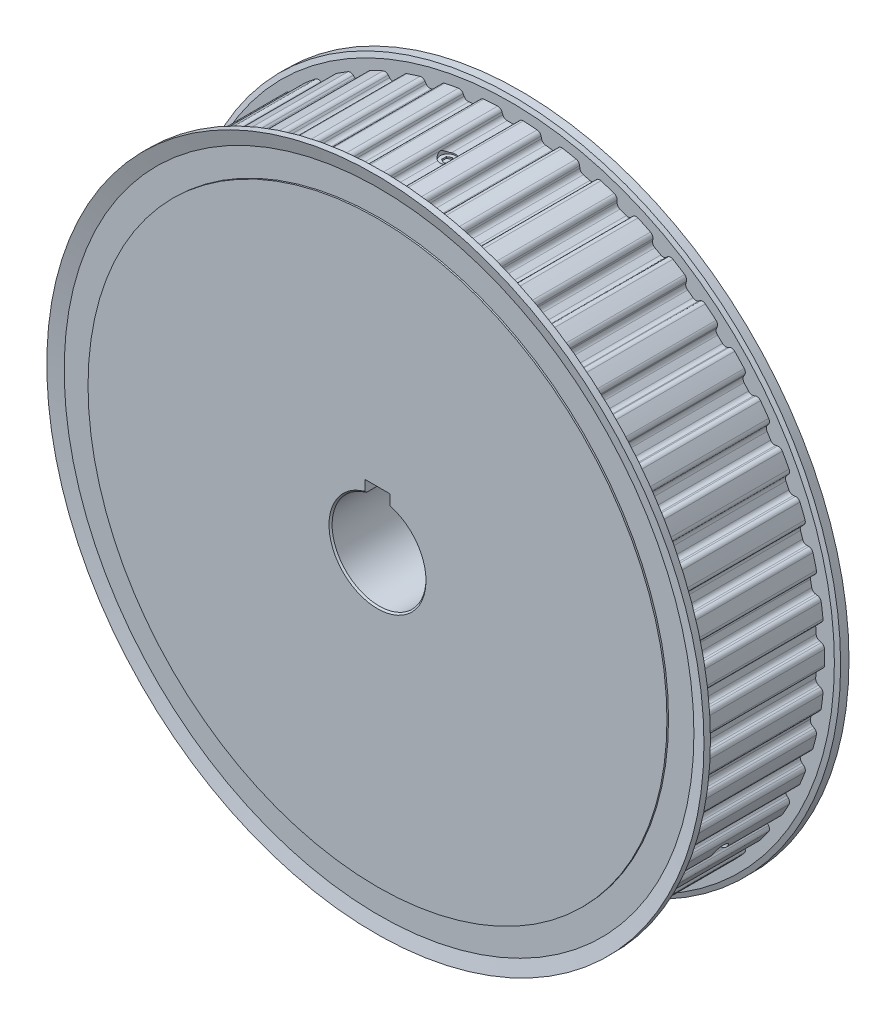
SolidWorks part; units mm, degrees
ref_plane "前视基准面" through (0, 0, 0) normal (0, 0, 1) x (1, 0, 0)
ref_plane "上视基准面" through (0, 0, 0) normal (0, 1, 0) x (1, 0, 0)
ref_plane "右视基准面" through (0, 0, 0) normal (1, 0, 0) x (0, 0, -1)
sketch "草图1" plane through (0, 0, 0) normal (1, 0, 0) x (0, 0, -1)
  line L0 (0, 0) -> (0, 92.5)
  line L1 (0, 92.5) -> (2.5, 92.5)
  line L2 (2.5, 92.5) -> (2.5, 102.38)
  line L3 (2.5, 102.38) -> (42.5, 102.38)
  line L4 (42.5, 102.38) -> (42.5, 92.5)
  line L5 (42.5, 92.5) -> (45, 92.5)
  line L6 (45, 92.5) -> (45, 0)
  line L7 (45, 0) -> (0, 0)
  line L8 (45, 0) -> (0, 0) construction
revolve "旋转1" add sketch "草图1" angle 360 about L8
sketch "草图2" plane through (0, 0, 0) normal (1, 0, 0) x (0, 0, -1)
  line L0 (0, 0) -> (0, 15.5)
  line L1 (0, 15.5) -> (0.5, 15)
  line L2 (0.5, 15) -> (44.5, 15)
  line L3 (44.5, 15) -> (45, 15.5)
  line L4 (45, 15.5) -> (45, 0)
  line L5 (45, 0) -> (0, 0)
  line L6 (45, 0) -> (0, 0) construction
revolve "切除-旋转1" cut sketch "草图2" angle 360 about L6
sketch "草图3" plane through (0, 0, 0) normal (1, 0, 0) x (0, 0, -1)
  line L0 (42.5, 103.5) -> (42.5, 92.5)
  line L1 (42.5, 92.5) -> (44.5, 92.5)
  line L2 (44.5, 92.5) -> (44.5, 105)
  line L3 (44.5, 105) -> (43, 105)
  line L4 (43, 105) -> (42.5, 103.5)
  line L5 (50, 0) -> (-50, 0) construction
revolve "旋转2" add sketch "草图3" angle 360 about L5
ref_plane "基准面1" through (0, 0, -22.5) normal (0, 0, 1) x (1, 0, 0)
sketch "草图4" plane through (0, 0, -22.5) normal (0, 0, 1) x (1, 0, 0)
  line L0 (-99.3369, -3.5434) -> (-98.7119, -3.7273)
  line L1 (-98.4007, -8.6739) -> (-98.9977, -8.9348)
  line L2 (-98.1095, -15.9657) -> (-97.4664, -16.0698)
  line L3 (-96.5376, -20.9384) -> (-97.0972, -21.272)
  line L4 (-95.3348, -28.1361) -> (-94.6838, -28.1589)
  line L5 (-93.1521, -32.8727) -> (-93.6655, -33.2738)
  line L6 (-91.0567, -39.8629) -> (-90.4079, -39.8039)
  line L7 (-88.2976, -44.2885) -> (-88.7566, -44.7508)
  line L8 (-85.3425, -50.961) -> (-84.7063, -50.8211)
  line L9 (-82.0505, -55.0059) -> (-82.448, -55.5221)
  line L10 (-78.2825, -61.2554) -> (-77.6687, -61.0369)
  line L11 (-74.5094, -64.8559) -> (-74.8391, -65.4178)
  line L12 (-69.9879, -70.5838) -> (-69.4064, -70.2901)
  line L13 (-65.7933, -73.683) -> (-66.0499, -74.2817)
  line L14 (-60.5895, -78.799) -> (-60.0494, -78.4347)
  line L15 (-56.0396, -81.348) -> (-56.2191, -81.9743)
  line L16 (-50.2356, -85.7715) -> (-49.7454, -85.3424)
  line L17 (-45.4021, -87.7302) -> (-45.5017, -88.374)
  line L18 (-39.0894, -91.3914) -> (-38.6569, -90.9042)
  line L19 (-34.0486, -92.7288) -> (-34.0667, -93.38)
  line L20 (-27.3268, -95.57) -> (-26.9588, -95.0324)
  line L21 (-22.1581, -96.265) -> (-22.0945, -96.9134)
  line L22 (-15.1333, -98.2413) -> (-14.8355, -97.6619)
  line L23 (-9.9181, -98.2831) -> (-9.7738, -98.9184)
  line L24 (-2.701, -99.3634) -> (-2.4782, -98.7512)
  line L25 (2.4782, -98.7512) -> (2.701, -99.3634)
  line L26 (9.7738, -98.9184) -> (9.9181, -98.2831)
  line L27 (14.8355, -97.6619) -> (15.1333, -98.2413)
  line L28 (22.0945, -96.9134) -> (22.1581, -96.265)
  line L29 (26.9588, -95.0324) -> (27.3268, -95.57)
  line L30 (34.0667, -93.38) -> (34.0486, -92.7288)
  line L31 (38.6569, -90.9042) -> (39.0894, -91.3914)
  line L32 (45.5017, -88.374) -> (45.4021, -87.7302)
  line L33 (49.7454, -85.3424) -> (50.2356, -85.7715)
  line L34 (56.2191, -81.9743) -> (56.0396, -81.348)
  line L35 (60.0494, -78.4347) -> (60.5895, -78.799)
  line L36 (66.0499, -74.2817) -> (65.7933, -73.683)
  line L37 (69.4064, -70.2901) -> (69.9879, -70.5838)
  line L38 (74.8391, -65.4178) -> (74.5094, -64.8559)
  line L39 (77.6687, -61.0369) -> (78.2825, -61.2554)
  line L40 (82.448, -55.5221) -> (82.0505, -55.0059)
  line L41 (84.7063, -50.8211) -> (85.3425, -50.961)
  line L42 (88.7566, -44.7508) -> (88.2976, -44.2885)
  line L43 (90.4079, -39.8039) -> (91.0567, -39.8629)
  line L44 (93.6655, -33.2738) -> (93.1521, -32.8727)
  line L45 (94.6838, -28.1589) -> (95.3348, -28.1361)
  line L46 (97.0972, -21.272) -> (96.5376, -20.9384)
  line L47 (97.4664, -16.0698) -> (98.1095, -15.9657)
  line L48 (98.9977, -8.9348) -> (98.4007, -8.6739)
  line L49 (98.7119, -3.7273) -> (99.3369, -3.5434)
  line L50 (99.3369, 3.5434) -> (98.7119, 3.7273)
  line L51 (98.4007, 8.6739) -> (98.9977, 8.9348)
  line L52 (98.1095, 15.9657) -> (97.4664, 16.0698)
  line L53 (96.5376, 20.9384) -> (97.0972, 21.272)
  line L54 (95.3348, 28.1361) -> (94.6838, 28.1589)
  line L55 (93.1521, 32.8727) -> (93.6655, 33.2738)
  line L56 (91.0567, 39.8629) -> (90.4079, 39.8039)
  line L57 (88.2976, 44.2885) -> (88.7566, 44.7508)
  line L58 (85.3425, 50.961) -> (84.7063, 50.8211)
  line L59 (82.0505, 55.0059) -> (82.448, 55.5221)
  line L60 (78.2825, 61.2554) -> (77.6687, 61.0369)
  line L61 (74.5094, 64.8559) -> (74.8391, 65.4178)
  line L62 (69.9879, 70.5838) -> (69.4064, 70.2901)
  line L63 (65.7933, 73.683) -> (66.0499, 74.2817)
  line L64 (60.5895, 78.799) -> (60.0494, 78.4347)
  line L65 (56.0396, 81.348) -> (56.2191, 81.9743)
  line L66 (50.2356, 85.7715) -> (49.7454, 85.3424)
  line L67 (45.4021, 87.7302) -> (45.5017, 88.374)
  line L68 (39.0894, 91.3914) -> (38.6569, 90.9042)
  line L69 (34.0486, 92.7288) -> (34.0667, 93.38)
  line L70 (27.3268, 95.57) -> (26.9588, 95.0324)
  line L71 (22.1581, 96.265) -> (22.0945, 96.9134)
  line L72 (15.1333, 98.2413) -> (14.8355, 97.6619)
  line L73 (9.9181, 98.2831) -> (9.7738, 98.9184)
  line L74 (2.701, 99.3634) -> (2.4782, 98.7512)
  line L75 (-2.4782, 98.7512) -> (-2.701, 99.3634)
  line L76 (-9.7738, 98.9184) -> (-9.9181, 98.2831)
  line L77 (-14.8355, 97.6619) -> (-15.1333, 98.2413)
  line L78 (-22.0945, 96.9134) -> (-22.1581, 96.265)
  line L79 (-26.9588, 95.0324) -> (-27.3268, 95.57)
  line L80 (-34.0667, 93.38) -> (-34.0486, 92.7288)
  line L81 (-38.6569, 90.9042) -> (-39.0894, 91.3914)
  line L82 (-45.5017, 88.374) -> (-45.4021, 87.7302)
  line L83 (-49.7454, 85.3424) -> (-50.2356, 85.7715)
  line L84 (-56.2191, 81.9743) -> (-56.0396, 81.348)
  line L85 (-60.0494, 78.4347) -> (-60.5895, 78.799)
  line L86 (-66.0499, 74.2817) -> (-65.7933, 73.683)
  line L87 (-69.4064, 70.2901) -> (-69.9879, 70.5838)
  line L88 (-74.8391, 65.4178) -> (-74.5094, 64.8559)
  line L89 (-77.6687, 61.0369) -> (-78.2825, 61.2554)
  line L90 (-82.448, 55.5221) -> (-82.0505, 55.0059)
  line L91 (-84.7063, 50.8211) -> (-85.3425, 50.961)
  line L92 (-88.7566, 44.7508) -> (-88.2976, 44.2885)
  line L93 (-90.4079, 39.8039) -> (-91.0567, 39.8629)
  line L94 (-93.6655, 33.2738) -> (-93.1521, 32.8727)
  line L95 (-94.6838, 28.1589) -> (-95.3348, 28.1361)
  line L96 (-97.0972, 21.272) -> (-96.5376, 20.9384)
  line L97 (-97.4664, 16.0698) -> (-98.1095, 15.9657)
  line L98 (-98.9977, 8.9348) -> (-98.4007, 8.6739)
  line L99 (-98.7119, 3.7273) -> (-99.3369, 3.5434)
  circle A0 centre (0, 0) radius 200.76
  arc A1 (-100.3556, 2.2125) -> (-100.3556, -2.2125) centre (0, 0) ccw
  arc A2 (-100.3556, -2.2125) -> (-99.3369, -3.5434) centre (-98.936, -2.1812) ccw
  arc A3 (-98.7119, -3.7273) -> (-97.6589, -5.0614) centre (-99.127, -5.1375) cw
  arc A4 (-97.6589, -5.0614) -> (-97.5232, -7.2184) centre (0, 0) ccw
  arc A5 (-97.5232, -7.2184) -> (-98.4007, -8.6739) centre (-98.9892, -7.3269) cw
  arc A6 (-98.9977, -8.9348) -> (-99.8416, -10.3829) centre (-98.4292, -10.236) ccw
  arc A7 (-99.8416, -10.3829) -> (-99.287, -14.7729) centre (0, 0) ccw
  arc A8 (-99.287, -14.7729) -> (-98.1095, -15.9657) centre (-97.8824, -14.5639) ccw
  arc A9 (-97.4664, -16.0698) -> (-96.2545, -17.2614) centre (-97.7014, -17.5209) cw
  arc A10 (-96.2545, -17.2614) -> (-95.8495, -19.3844) centre (0, 0) ccw
  arc A11 (-95.8495, -19.3844) -> (-96.5376, -20.9384) centre (-97.2903, -19.6758) cw
  arc A12 (-97.0972, -21.272) -> (-97.753, -22.8145) centre (-96.3701, -22.4917) ccw
  arc A13 (-97.753, -22.8145) -> (-96.6525, -27.1004) centre (0, 0) ccw
  arc A14 (-96.6525, -27.1004) -> (-95.3348, -28.1361) centre (-95.2853, -26.717) ccw
  arc A15 (-94.6838, -28.1589) -> (-93.3321, -29.1892) centre (-94.7351, -29.628) cw
  arc A16 (-93.3321, -29.1892) -> (-92.6642, -31.2446) centre (0, 0) ccw
  arc A17 (-92.6642, -31.2446) -> (-93.1521, -32.8727) centre (-94.0572, -31.7143) cw
  arc A18 (-93.6655, -33.2738) -> (-94.1228, -34.8863) centre (-92.7913, -34.3928) ccw
  arc A19 (-94.1228, -34.8863) -> (-92.4938, -39.0005) centre (0, 0) ccw
  arc A20 (-92.4938, -39.0005) -> (-91.0567, -39.8629) centre (-91.1854, -38.4487) ccw
  arc A21 (-90.4079, -39.8039) -> (-88.9377, -40.6566) centre (-90.2747, -41.2678) cw
  arc A22 (-88.9377, -40.6566) -> (-88.0175, -42.6122) centre (0, 0) ccw
  arc A23 (-88.0175, -42.6122) -> (-88.2976, -44.2885) centre (-89.3406, -43.2527) cw
  arc A24 (-88.7566, -44.7508) -> (-89.0082, -46.4079) centre (-87.749, -45.7514) ccw
  arc A25 (-89.0082, -46.4079) -> (-86.8764, -50.2855) centre (0, 0) ccw
  arc A26 (-86.8764, -50.2855) -> (-85.3425, -50.961) centre (-85.6475, -49.5741) ccw
  arc A27 (-84.7063, -50.8211) -> (-83.1408, -51.4829) centre (-84.3906, -52.2568) cw
  arc A28 (-83.1408, -51.4829) -> (-81.9828, -53.3077) centre (0, 0) ccw
  arc A29 (-81.9828, -53.3077) -> (-82.0505, -55.0059) centre (-83.2151, -54.109) cw
  arc A30 (-82.448, -55.5221) -> (-82.4898, -57.1976) centre (-81.3229, -56.3885) ccw
  arc A31 (-82.4898, -57.1976) -> (-79.8889, -60.7775) centre (0, 0) ccw
  arc A32 (-79.8889, -60.7775) -> (-78.2825, -61.2554) centre (-78.7588, -59.9177) ccw
  arc A33 (-77.6687, -61.0369) -> (-76.0327, -61.4973) centre (-77.1756, -62.4217) cw
  arc A34 (-76.0327, -61.4973) -> (-74.6551, -63.1625) centre (0, 0) ccw
  arc A35 (-74.6551, -63.1625) -> (-74.5094, -64.8559) centre (-75.7773, -64.112) cw
  arc A36 (-74.8391, -65.4178) -> (-74.6706, -67.0853) centre (-73.6143, -66.1363) ccw
  arc A37 (-74.6706, -67.0853) -> (-71.6416, -70.311) centre (0, 0) ccw
  arc A38 (-71.6416, -70.311) -> (-69.9879, -70.5838) centre (-70.6281, -69.3163) ccw
  arc A39 (-69.4064, -70.2901) -> (-67.7255, -70.5418) centre (-68.7436, -71.6022) cw
  arc A40 (-67.7255, -70.5418) -> (-66.15, -72.0212) centre (0, 0) ccw
  arc A41 (-66.15, -72.0212) -> (-65.7933, -73.683) centre (-67.1444, -73.1039) cw
  arc A42 (-66.0499, -74.2817) -> (-65.6738, -75.9151) centre (-64.7448, -74.8411) ccw
  arc A43 (-65.6738, -75.9151) -> (-62.2643, -78.7356) centre (0, 0) ccw
  arc A44 (-62.2643, -78.7356) -> (-60.5895, -78.799) centre (-61.3835, -77.6218) ccw
  arc A45 (-60.0494, -78.4347) -> (-58.3502, -78.4738) centre (-59.2274, -79.6534) cw
  arc A46 (-58.3502, -78.4738) -> (-56.6018, -79.7441) centre (0, 0) ccw
  arc A47 (-56.6018, -79.7441) -> (-56.0396, -81.348) centre (-57.4526, -80.9428) cw
  arc A48 (-56.2191, -81.9743) -> (-55.6413, -83.5476) centre (-54.8542, -82.3657) ccw
  arc A49 (-55.6413, -83.5476) -> (-51.9052, -85.9185) centre (0, 0) ccw
  arc A50 (-51.9052, -85.9185) -> (-50.2356, -85.7715) centre (-51.1709, -84.7031) ccw
  arc A51 (-49.7454, -85.3424) -> (-48.0548, -85.1682) centre (-48.7771, -86.4485) cw
  arc A52 (-48.0548, -85.1682) -> (-46.1609, -86.2094) centre (0, 0) ccw
  arc A53 (-46.1609, -86.2094) -> (-45.4021, -87.7302) centre (-46.8548, -87.5053) cw
  arc A54 (-45.5017, -88.374) -> (-44.7312, -89.8625) centre (-44.0985, -88.5912) ccw
  arc A55 (-44.7312, -89.8625) -> (-40.7275, -91.7465) centre (0, 0) ccw
  arc A56 (-40.7275, -91.7465) -> (-39.0894, -91.3914) centre (-40.1513, -90.4486) ccw
  arc A57 (-38.6569, -90.9042) -> (-37.0014, -90.5195) centre (-37.5576, -91.8802) cw
  arc A58 (-37.0014, -90.5195) -> (-34.992, -91.3151) centre (0, 0) ccw
  arc A59 (-34.992, -91.3151) -> (-34.0486, -92.7288) centre (-35.518, -92.6878) cw
  arc A60 (-34.0667, -93.38) -> (-33.1158, -94.7602) centre (-32.6473, -93.4197) ccw
  arc A61 (-33.1158, -94.7602) -> (-28.9074, -96.1275) centre (0, 0) ccw
  arc A62 (-28.9074, -96.1275) -> (-27.3268, -95.57) centre (-28.4985, -94.7677) ccw
  arc A63 (-26.9588, -95.0324) -> (-25.3646, -94.4432) centre (-25.7458, -95.8629) cw
  arc A64 (-25.3646, -94.4432) -> (-23.2712, -94.9807) centre (0, 0) ccw
  arc A65 (-23.2712, -94.9807) -> (-22.1581, -96.265) centre (-23.6211, -96.4085) cw
  arc A66 (-22.0945, -96.9134) -> (-20.978, -98.1635) centre (-20.6813, -96.7748) ccw
  arc A67 (-20.978, -98.1635) -> (-16.6315, -98.9926) centre (0, 0) ccw
  arc A68 (-16.6315, -98.9926) -> (-15.1333, -98.2413) centre (-16.3962, -97.5922) ccw
  arc A69 (-14.8355, -97.6619) -> (-13.3277, -96.8775) centre (-13.528, -98.3338) cw
  arc A70 (-13.3277, -96.8775) -> (-11.1835, -97.1484) centre (0, 0) ccw
  arc A71 (-11.1835, -97.1484) -> (-9.9181, -98.2831) centre (-11.3516, -98.6088) cw
  arc A72 (-9.7738, -98.9184) -> (-8.5095, -100.0187) centre (-8.3891, -98.6038) ccw
  arc A73 (-8.5095, -100.0187) -> (-4.0933, -100.2965) centre (0, 0) ccw
  arc A74 (-4.0933, -100.2965) -> (-2.701, -99.3634) centre (-4.0354, -98.8777) ccw
  arc A75 (-2.4782, -98.7512) -> (-1.0806, -97.784) centre (-1.0969, -99.2539) cw
  arc A76 (-1.0806, -97.784) -> (1.0806, -97.784) centre (0, 0) ccw
  arc A77 (1.0806, -97.784) -> (2.4782, -98.7512) centre (1.0969, -99.2539) cw
  arc A78 (2.701, -99.3634) -> (4.0933, -100.2965) centre (4.0354, -98.8777) ccw
  arc A79 (4.0933, -100.2965) -> (8.5095, -100.0187) centre (0, 0) ccw
  arc A80 (8.5095, -100.0187) -> (9.7738, -98.9184) centre (8.3891, -98.6038) ccw
  arc A81 (9.9181, -98.2831) -> (11.1835, -97.1484) centre (11.3516, -98.6088) cw
  arc A82 (11.1835, -97.1484) -> (13.3277, -96.8775) centre (0, 0) ccw
  arc A83 (13.3277, -96.8775) -> (14.8355, -97.6619) centre (13.528, -98.3338) cw
  arc A84 (15.1333, -98.2413) -> (16.6315, -98.9926) centre (16.3962, -97.5922) ccw
  arc A85 (16.6315, -98.9926) -> (20.978, -98.1635) centre (0, 0) ccw
  arc A86 (20.978, -98.1635) -> (22.0945, -96.9134) centre (20.6813, -96.7748) ccw
  arc A87 (22.1581, -96.265) -> (23.2712, -94.9807) centre (23.6211, -96.4085) cw
  arc A88 (23.2712, -94.9807) -> (25.3646, -94.4432) centre (0, 0) ccw
  arc A89 (25.3646, -94.4432) -> (26.9588, -95.0324) centre (25.7458, -95.8629) cw
  arc A90 (27.3268, -95.57) -> (28.9074, -96.1275) centre (28.4985, -94.7677) ccw
  arc A91 (28.9074, -96.1275) -> (33.1158, -94.7602) centre (0, 0) ccw
  arc A92 (33.1158, -94.7602) -> (34.0667, -93.38) centre (32.6473, -93.4197) ccw
  arc A93 (34.0486, -92.7288) -> (34.992, -91.3151) centre (35.518, -92.6878) cw
  arc A94 (34.992, -91.3151) -> (37.0014, -90.5195) centre (0, 0) ccw
  arc A95 (37.0014, -90.5195) -> (38.6569, -90.9042) centre (37.5576, -91.8802) cw
  arc A96 (39.0894, -91.3914) -> (40.7275, -91.7465) centre (40.1513, -90.4486) ccw
  arc A97 (40.7275, -91.7465) -> (44.7312, -89.8625) centre (0, 0) ccw
  arc A98 (44.7312, -89.8625) -> (45.5017, -88.374) centre (44.0985, -88.5912) ccw
  arc A99 (45.4021, -87.7302) -> (46.1609, -86.2094) centre (46.8548, -87.5053) cw
  arc A100 (46.1609, -86.2094) -> (48.0548, -85.1682) centre (0, 0) ccw
  arc A101 (48.0548, -85.1682) -> (49.7454, -85.3424) centre (48.7771, -86.4485) cw
  arc A102 (50.2356, -85.7715) -> (51.9052, -85.9185) centre (51.1709, -84.7031) ccw
  arc A103 (51.9052, -85.9185) -> (55.6413, -83.5476) centre (0, 0) ccw
  arc A104 (55.6413, -83.5476) -> (56.2191, -81.9743) centre (54.8542, -82.3657) ccw
  arc A105 (56.0396, -81.348) -> (56.6018, -79.7441) centre (57.4526, -80.9428) cw
  arc A106 (56.6018, -79.7441) -> (58.3502, -78.4738) centre (0, 0) ccw
  arc A107 (58.3502, -78.4738) -> (60.0494, -78.4347) centre (59.2274, -79.6534) cw
  arc A108 (60.5895, -78.799) -> (62.2643, -78.7356) centre (61.3835, -77.6218) ccw
  arc A109 (62.2643, -78.7356) -> (65.6738, -75.9151) centre (0, 0) ccw
  arc A110 (65.6738, -75.9151) -> (66.0499, -74.2817) centre (64.7448, -74.8411) ccw
  arc A111 (65.7933, -73.683) -> (66.15, -72.0212) centre (67.1444, -73.1039) cw
  arc A112 (66.15, -72.0212) -> (67.7255, -70.5418) centre (0, 0) ccw
  arc A113 (67.7255, -70.5418) -> (69.4064, -70.2901) centre (68.7436, -71.6022) cw
  arc A114 (69.9879, -70.5838) -> (71.6416, -70.311) centre (70.6281, -69.3163) ccw
  arc A115 (71.6416, -70.311) -> (74.6706, -67.0853) centre (0, 0) ccw
  arc A116 (74.6706, -67.0853) -> (74.8391, -65.4178) centre (73.6143, -66.1363) ccw
  arc A117 (74.5094, -64.8559) -> (74.6551, -63.1625) centre (75.7773, -64.112) cw
  arc A118 (74.6551, -63.1625) -> (76.0327, -61.4973) centre (0, 0) ccw
  arc A119 (76.0327, -61.4973) -> (77.6687, -61.0369) centre (77.1756, -62.4217) cw
  arc A120 (78.2825, -61.2554) -> (79.8889, -60.7775) centre (78.7588, -59.9177) ccw
  arc A121 (79.8889, -60.7775) -> (82.4898, -57.1976) centre (0, 0) ccw
  arc A122 (82.4898, -57.1976) -> (82.448, -55.5221) centre (81.3229, -56.3885) ccw
  arc A123 (82.0505, -55.0059) -> (81.9828, -53.3077) centre (83.2151, -54.109) cw
  arc A124 (81.9828, -53.3077) -> (83.1408, -51.4829) centre (0, 0) ccw
  arc A125 (83.1408, -51.4829) -> (84.7063, -50.8211) centre (84.3906, -52.2568) cw
  arc A126 (85.3425, -50.961) -> (86.8764, -50.2855) centre (85.6475, -49.5741) ccw
  arc A127 (86.8764, -50.2855) -> (89.0082, -46.4079) centre (0, 0) ccw
  arc A128 (89.0082, -46.4079) -> (88.7566, -44.7508) centre (87.749, -45.7514) ccw
  arc A129 (88.2976, -44.2885) -> (88.0175, -42.6122) centre (89.3406, -43.2527) cw
  arc A130 (88.0175, -42.6122) -> (88.9377, -40.6566) centre (0, 0) ccw
  arc A131 (88.9377, -40.6566) -> (90.4079, -39.8039) centre (90.2747, -41.2678) cw
  arc A132 (91.0567, -39.8629) -> (92.4938, -39.0005) centre (91.1854, -38.4487) ccw
  arc A133 (92.4938, -39.0005) -> (94.1228, -34.8863) centre (0, 0) ccw
  arc A134 (94.1228, -34.8863) -> (93.6655, -33.2738) centre (92.7913, -34.3928) ccw
  arc A135 (93.1521, -32.8727) -> (92.6642, -31.2446) centre (94.0572, -31.7143) cw
  arc A136 (92.6642, -31.2446) -> (93.3321, -29.1892) centre (0, 0) ccw
  arc A137 (93.3321, -29.1892) -> (94.6838, -28.1589) centre (94.7351, -29.628) cw
  arc A138 (95.3348, -28.1361) -> (96.6525, -27.1004) centre (95.2853, -26.717) ccw
  arc A139 (96.6525, -27.1004) -> (97.753, -22.8145) centre (0, 0) ccw
  arc A140 (97.753, -22.8145) -> (97.0972, -21.272) centre (96.3701, -22.4917) ccw
  arc A141 (96.5376, -20.9384) -> (95.8495, -19.3844) centre (97.2903, -19.6758) cw
  arc A142 (95.8495, -19.3844) -> (96.2545, -17.2614) centre (0, 0) ccw
  arc A143 (96.2545, -17.2614) -> (97.4664, -16.0698) centre (97.7014, -17.5209) cw
  arc A144 (98.1095, -15.9657) -> (99.287, -14.7729) centre (97.8824, -14.5639) ccw
  arc A145 (99.287, -14.7729) -> (99.8416, -10.3829) centre (0, 0) ccw
  arc A146 (99.8416, -10.3829) -> (98.9977, -8.9348) centre (98.4292, -10.236) ccw
  arc A147 (98.4007, -8.6739) -> (97.5232, -7.2184) centre (98.9892, -7.3269) cw
  arc A148 (97.5232, -7.2184) -> (97.6589, -5.0614) centre (0, 0) ccw
  arc A149 (97.6589, -5.0614) -> (98.7119, -3.7273) centre (99.127, -5.1375) cw
  arc A150 (99.3369, -3.5434) -> (100.3556, -2.2125) centre (98.936, -2.1812) ccw
  arc A151 (100.3556, -2.2125) -> (100.3556, 2.2125) centre (0, 0) ccw
  arc A152 (100.3556, 2.2125) -> (99.3369, 3.5434) centre (98.936, 2.1812) ccw
  arc A153 (98.7119, 3.7273) -> (97.6589, 5.0614) centre (99.127, 5.1375) cw
  arc A154 (97.6589, 5.0614) -> (97.5232, 7.2184) centre (0, 0) ccw
  arc A155 (97.5232, 7.2184) -> (98.4007, 8.6739) centre (98.9892, 7.3269) cw
  arc A156 (98.9977, 8.9348) -> (99.8416, 10.3829) centre (98.4292, 10.236) ccw
  arc A157 (99.8416, 10.3829) -> (99.287, 14.7729) centre (0, 0) ccw
  arc A158 (99.287, 14.7729) -> (98.1095, 15.9657) centre (97.8824, 14.5639) ccw
  arc A159 (97.4664, 16.0698) -> (96.2545, 17.2614) centre (97.7014, 17.5209) cw
  arc A160 (96.2545, 17.2614) -> (95.8495, 19.3844) centre (0, 0) ccw
  arc A161 (95.8495, 19.3844) -> (96.5376, 20.9384) centre (97.2903, 19.6758) cw
  arc A162 (97.0972, 21.272) -> (97.753, 22.8145) centre (96.3701, 22.4917) ccw
  arc A163 (97.753, 22.8145) -> (96.6525, 27.1004) centre (0, 0) ccw
  arc A164 (96.6525, 27.1004) -> (95.3348, 28.1361) centre (95.2853, 26.717) ccw
  arc A165 (94.6838, 28.1589) -> (93.3321, 29.1892) centre (94.7351, 29.628) cw
  arc A166 (93.3321, 29.1892) -> (92.6642, 31.2446) centre (0, 0) ccw
  arc A167 (92.6642, 31.2446) -> (93.1521, 32.8727) centre (94.0572, 31.7143) cw
  arc A168 (93.6655, 33.2738) -> (94.1228, 34.8863) centre (92.7913, 34.3928) ccw
  arc A169 (94.1228, 34.8863) -> (92.4938, 39.0005) centre (0, 0) ccw
  arc A170 (92.4938, 39.0005) -> (91.0567, 39.8629) centre (91.1854, 38.4487) ccw
  arc A171 (90.4079, 39.8039) -> (88.9377, 40.6566) centre (90.2747, 41.2678) cw
  arc A172 (88.9377, 40.6566) -> (88.0175, 42.6122) centre (0, 0) ccw
  arc A173 (88.0175, 42.6122) -> (88.2976, 44.2885) centre (89.3406, 43.2527) cw
  arc A174 (88.7566, 44.7508) -> (89.0082, 46.4079) centre (87.749, 45.7514) ccw
  arc A175 (89.0082, 46.4079) -> (86.8764, 50.2855) centre (0, 0) ccw
  arc A176 (86.8764, 50.2855) -> (85.3425, 50.961) centre (85.6475, 49.5741) ccw
  arc A177 (84.7063, 50.8211) -> (83.1408, 51.4829) centre (84.3906, 52.2568) cw
  arc A178 (83.1408, 51.4829) -> (81.9828, 53.3077) centre (0, 0) ccw
  arc A179 (81.9828, 53.3077) -> (82.0505, 55.0059) centre (83.2151, 54.109) cw
  arc A180 (82.448, 55.5221) -> (82.4898, 57.1976) centre (81.3229, 56.3885) ccw
  arc A181 (82.4898, 57.1976) -> (79.8889, 60.7775) centre (0, 0) ccw
  arc A182 (79.8889, 60.7775) -> (78.2825, 61.2554) centre (78.7588, 59.9177) ccw
  arc A183 (77.6687, 61.0369) -> (76.0327, 61.4973) centre (77.1756, 62.4217) cw
  arc A184 (76.0327, 61.4973) -> (74.6551, 63.1625) centre (0, 0) ccw
  arc A185 (74.6551, 63.1625) -> (74.5094, 64.8559) centre (75.7773, 64.112) cw
  arc A186 (74.8391, 65.4178) -> (74.6706, 67.0853) centre (73.6143, 66.1363) ccw
  arc A187 (74.6706, 67.0853) -> (71.6416, 70.311) centre (0, 0) ccw
  arc A188 (71.6416, 70.311) -> (69.9879, 70.5838) centre (70.6281, 69.3163) ccw
  arc A189 (69.4064, 70.2901) -> (67.7255, 70.5418) centre (68.7436, 71.6022) cw
  arc A190 (67.7255, 70.5418) -> (66.15, 72.0212) centre (0, 0) ccw
  arc A191 (66.15, 72.0212) -> (65.7933, 73.683) centre (67.1444, 73.1039) cw
  arc A192 (66.0499, 74.2817) -> (65.6738, 75.9151) centre (64.7448, 74.8411) ccw
  arc A193 (65.6738, 75.9151) -> (62.2643, 78.7356) centre (0, 0) ccw
  arc A194 (62.2643, 78.7356) -> (60.5895, 78.799) centre (61.3835, 77.6218) ccw
  arc A195 (60.0494, 78.4347) -> (58.3502, 78.4738) centre (59.2274, 79.6534) cw
  arc A196 (58.3502, 78.4738) -> (56.6018, 79.7441) centre (0, 0) ccw
  arc A197 (56.6018, 79.7441) -> (56.0396, 81.348) centre (57.4526, 80.9428) cw
  arc A198 (56.2191, 81.9743) -> (55.6413, 83.5476) centre (54.8542, 82.3657) ccw
  arc A199 (55.6413, 83.5476) -> (51.9052, 85.9185) centre (0, 0) ccw
  arc A200 (51.9052, 85.9185) -> (50.2356, 85.7715) centre (51.1709, 84.7031) ccw
  arc A201 (49.7454, 85.3424) -> (48.0548, 85.1682) centre (48.7771, 86.4485) cw
  arc A202 (48.0548, 85.1682) -> (46.1609, 86.2094) centre (0, 0) ccw
  arc A203 (46.1609, 86.2094) -> (45.4021, 87.7302) centre (46.8548, 87.5053) cw
  arc A204 (45.5017, 88.374) -> (44.7312, 89.8625) centre (44.0985, 88.5912) ccw
  arc A205 (44.7312, 89.8625) -> (40.7275, 91.7465) centre (0, 0) ccw
  arc A206 (40.7275, 91.7465) -> (39.0894, 91.3914) centre (40.1513, 90.4486) ccw
  arc A207 (38.6569, 90.9042) -> (37.0014, 90.5195) centre (37.5576, 91.8802) cw
  arc A208 (37.0014, 90.5195) -> (34.992, 91.3151) centre (0, 0) ccw
  arc A209 (34.992, 91.3151) -> (34.0486, 92.7288) centre (35.518, 92.6878) cw
  arc A210 (34.0667, 93.38) -> (33.1158, 94.7602) centre (32.6473, 93.4197) ccw
  arc A211 (33.1158, 94.7602) -> (28.9074, 96.1275) centre (0, 0) ccw
  arc A212 (28.9074, 96.1275) -> (27.3268, 95.57) centre (28.4985, 94.7677) ccw
  arc A213 (26.9588, 95.0324) -> (25.3646, 94.4432) centre (25.7458, 95.8629) cw
  arc A214 (25.3646, 94.4432) -> (23.2712, 94.9807) centre (0, 0) ccw
  arc A215 (23.2712, 94.9807) -> (22.1581, 96.265) centre (23.6211, 96.4085) cw
  arc A216 (22.0945, 96.9134) -> (20.978, 98.1635) centre (20.6813, 96.7748) ccw
  arc A217 (20.978, 98.1635) -> (16.6315, 98.9926) centre (0, 0) ccw
  arc A218 (16.6315, 98.9926) -> (15.1333, 98.2413) centre (16.3962, 97.5922) ccw
  arc A219 (14.8355, 97.6619) -> (13.3277, 96.8775) centre (13.528, 98.3338) cw
  arc A220 (13.3277, 96.8775) -> (11.1835, 97.1484) centre (0, 0) ccw
  arc A221 (11.1835, 97.1484) -> (9.9181, 98.2831) centre (11.3516, 98.6088) cw
  arc A222 (9.7738, 98.9184) -> (8.5095, 100.0187) centre (8.3891, 98.6038) ccw
  arc A223 (8.5095, 100.0187) -> (4.0933, 100.2965) centre (0, 0) ccw
  arc A224 (4.0933, 100.2965) -> (2.701, 99.3634) centre (4.0354, 98.8777) ccw
  arc A225 (2.4782, 98.7512) -> (1.0806, 97.784) centre (1.0969, 99.2539) cw
  arc A226 (1.0806, 97.784) -> (-1.0806, 97.784) centre (0, 0) ccw
  arc A227 (-1.0806, 97.784) -> (-2.4782, 98.7512) centre (-1.0969, 99.2539) cw
  arc A228 (-2.701, 99.3634) -> (-4.0933, 100.2965) centre (-4.0354, 98.8777) ccw
  arc A229 (-4.0933, 100.2965) -> (-8.5095, 100.0187) centre (0, 0) ccw
  arc A230 (-8.5095, 100.0187) -> (-9.7738, 98.9184) centre (-8.3891, 98.6038) ccw
  arc A231 (-9.9181, 98.2831) -> (-11.1835, 97.1484) centre (-11.3516, 98.6088) cw
  arc A232 (-11.1835, 97.1484) -> (-13.3277, 96.8775) centre (0, 0) ccw
  arc A233 (-13.3277, 96.8775) -> (-14.8355, 97.6619) centre (-13.528, 98.3338) cw
  arc A234 (-15.1333, 98.2413) -> (-16.6315, 98.9926) centre (-16.3962, 97.5922) ccw
  arc A235 (-16.6315, 98.9926) -> (-20.978, 98.1635) centre (0, 0) ccw
  arc A236 (-20.978, 98.1635) -> (-22.0945, 96.9134) centre (-20.6813, 96.7748) ccw
  arc A237 (-22.1581, 96.265) -> (-23.2712, 94.9807) centre (-23.6211, 96.4085) cw
  arc A238 (-23.2712, 94.9807) -> (-25.3646, 94.4432) centre (0, 0) ccw
  arc A239 (-25.3646, 94.4432) -> (-26.9588, 95.0324) centre (-25.7458, 95.8629) cw
  arc A240 (-27.3268, 95.57) -> (-28.9074, 96.1275) centre (-28.4985, 94.7677) ccw
  arc A241 (-28.9074, 96.1275) -> (-33.1158, 94.7602) centre (0, 0) ccw
  arc A242 (-33.1158, 94.7602) -> (-34.0667, 93.38) centre (-32.6473, 93.4197) ccw
  arc A243 (-34.0486, 92.7288) -> (-34.992, 91.3151) centre (-35.518, 92.6878) cw
  arc A244 (-34.992, 91.3151) -> (-37.0014, 90.5195) centre (0, 0) ccw
  arc A245 (-37.0014, 90.5195) -> (-38.6569, 90.9042) centre (-37.5576, 91.8802) cw
  arc A246 (-39.0894, 91.3914) -> (-40.7275, 91.7465) centre (-40.1513, 90.4486) ccw
  arc A247 (-40.7275, 91.7465) -> (-44.7312, 89.8625) centre (0, 0) ccw
  arc A248 (-44.7312, 89.8625) -> (-45.5017, 88.374) centre (-44.0985, 88.5912) ccw
  arc A249 (-45.4021, 87.7302) -> (-46.1609, 86.2094) centre (-46.8548, 87.5053) cw
  arc A250 (-46.1609, 86.2094) -> (-48.0548, 85.1682) centre (0, 0) ccw
  arc A251 (-48.0548, 85.1682) -> (-49.7454, 85.3424) centre (-48.7771, 86.4485) cw
  arc A252 (-50.2356, 85.7715) -> (-51.9052, 85.9185) centre (-51.1709, 84.7031) ccw
  arc A253 (-51.9052, 85.9185) -> (-55.6413, 83.5476) centre (0, 0) ccw
  arc A254 (-55.6413, 83.5476) -> (-56.2191, 81.9743) centre (-54.8542, 82.3657) ccw
  arc A255 (-56.0396, 81.348) -> (-56.6018, 79.7441) centre (-57.4526, 80.9428) cw
  arc A256 (-56.6018, 79.7441) -> (-58.3502, 78.4738) centre (0, 0) ccw
  arc A257 (-58.3502, 78.4738) -> (-60.0494, 78.4347) centre (-59.2274, 79.6534) cw
  arc A258 (-60.5895, 78.799) -> (-62.2643, 78.7356) centre (-61.3835, 77.6218) ccw
  arc A259 (-62.2643, 78.7356) -> (-65.6738, 75.9151) centre (0, 0) ccw
  arc A260 (-65.6738, 75.9151) -> (-66.0499, 74.2817) centre (-64.7448, 74.8411) ccw
  arc A261 (-65.7933, 73.683) -> (-66.15, 72.0212) centre (-67.1444, 73.1039) cw
  arc A262 (-66.15, 72.0212) -> (-67.7255, 70.5418) centre (0, 0) ccw
  arc A263 (-67.7255, 70.5418) -> (-69.4064, 70.2901) centre (-68.7436, 71.6022) cw
  arc A264 (-69.9879, 70.5838) -> (-71.6416, 70.311) centre (-70.6281, 69.3163) ccw
  arc A265 (-71.6416, 70.311) -> (-74.6706, 67.0853) centre (0, 0) ccw
  arc A266 (-74.6706, 67.0853) -> (-74.8391, 65.4178) centre (-73.6143, 66.1363) ccw
  arc A267 (-74.5094, 64.8559) -> (-74.6551, 63.1625) centre (-75.7773, 64.112) cw
  arc A268 (-74.6551, 63.1625) -> (-76.0327, 61.4973) centre (0, 0) ccw
  arc A269 (-76.0327, 61.4973) -> (-77.6687, 61.0369) centre (-77.1756, 62.4217) cw
  arc A270 (-78.2825, 61.2554) -> (-79.8889, 60.7775) centre (-78.7588, 59.9177) ccw
  arc A271 (-79.8889, 60.7775) -> (-82.4898, 57.1976) centre (0, 0) ccw
  arc A272 (-82.4898, 57.1976) -> (-82.448, 55.5221) centre (-81.3229, 56.3885) ccw
  arc A273 (-82.0505, 55.0059) -> (-81.9828, 53.3077) centre (-83.2151, 54.109) cw
  arc A274 (-81.9828, 53.3077) -> (-83.1408, 51.4829) centre (0, 0) ccw
  arc A275 (-83.1408, 51.4829) -> (-84.7063, 50.8211) centre (-84.3906, 52.2568) cw
  arc A276 (-85.3425, 50.961) -> (-86.8764, 50.2855) centre (-85.6475, 49.5741) ccw
  arc A277 (-86.8764, 50.2855) -> (-89.0082, 46.4079) centre (0, 0) ccw
  arc A278 (-89.0082, 46.4079) -> (-88.7566, 44.7508) centre (-87.749, 45.7514) ccw
  arc A279 (-88.2976, 44.2885) -> (-88.0175, 42.6122) centre (-89.3406, 43.2527) cw
  arc A280 (-88.0175, 42.6122) -> (-88.9377, 40.6566) centre (0, 0) ccw
  arc A281 (-88.9377, 40.6566) -> (-90.4079, 39.8039) centre (-90.2747, 41.2678) cw
  arc A282 (-91.0567, 39.8629) -> (-92.4938, 39.0005) centre (-91.1854, 38.4487) ccw
  arc A283 (-92.4938, 39.0005) -> (-94.1228, 34.8863) centre (0, 0) ccw
  arc A284 (-94.1228, 34.8863) -> (-93.6655, 33.2738) centre (-92.7913, 34.3928) ccw
  arc A285 (-93.1521, 32.8727) -> (-92.6642, 31.2446) centre (-94.0572, 31.7143) cw
  arc A286 (-92.6642, 31.2446) -> (-93.3321, 29.1892) centre (0, 0) ccw
  arc A287 (-93.3321, 29.1892) -> (-94.6838, 28.1589) centre (-94.7351, 29.628) cw
  arc A288 (-95.3348, 28.1361) -> (-96.6525, 27.1004) centre (-95.2853, 26.717) ccw
  arc A289 (-96.6525, 27.1004) -> (-97.753, 22.8145) centre (0, 0) ccw
  arc A290 (-97.753, 22.8145) -> (-97.0972, 21.272) centre (-96.3701, 22.4917) ccw
  arc A291 (-96.5376, 20.9384) -> (-95.8495, 19.3844) centre (-97.2903, 19.6758) cw
  arc A292 (-95.8495, 19.3844) -> (-96.2545, 17.2614) centre (0, 0) ccw
  arc A293 (-96.2545, 17.2614) -> (-97.4664, 16.0698) centre (-97.7014, 17.5209) cw
  arc A294 (-98.1095, 15.9657) -> (-99.287, 14.7729) centre (-97.8824, 14.5639) ccw
  arc A295 (-99.287, 14.7729) -> (-99.8416, 10.3829) centre (0, 0) ccw
  arc A296 (-99.8416, 10.3829) -> (-98.9977, 8.9348) centre (-98.4292, 10.236) ccw
  arc A297 (-98.4007, 8.6739) -> (-97.5232, 7.2184) centre (-98.9892, 7.3269) cw
  arc A298 (-97.5232, 7.2184) -> (-97.6589, 5.0614) centre (0, 0) ccw
  arc A299 (-97.6589, 5.0614) -> (-98.7119, 3.7273) centre (-99.127, 5.1375) cw
  arc A300 (-99.3369, 3.5434) -> (-100.3556, 2.2125) centre (-98.936, 2.1812) ccw
extrude "切除-拉伸1" cut sketch "草图4" along normal blind 20 and the other way blind 20
sketch "草图5" plane through (0, 0, -22.5) normal (0, 0, 1) x (1, 0, 0)
  line L0 (86.9403, -50.195) -> (85.711, -52.3241)
  line L1 (85.711, -52.3241) -> (10.9038, -9.1341)
  line L2 (10.9038, -9.1341) -> (12.133, -7.005)
  line L3 (12.133, -7.005) -> (86.9403, -50.195)
  line L4 (12.133, -7.005) -> (86.9403, -50.195) construction
revolve "切除-旋转2" cut sketch "草图5" angle 360 about L4
ref_plane "基准面2" through (0, 97.38, 0) normal (0, 1, 0) x (1, 0, 0)
sketch "草图6" plane through (0, 0, -22.5) normal (0, 0, 1) x (1, 0, 0)
  line L0 (84.3336, -48.69) -> (82.8336, -51.2881)
  line L1 (82.8336, -51.2881) -> (12.3564, -10.5981)
  line L2 (12.3564, -10.5981) -> (13.8564, -8)
  line L3 (13.8564, -8) -> (84.3336, -48.69)
  line L4 (13.8564, -8) -> (84.3336, -48.69) construction
revolve "旋转3" add sketch "草图6" angle 360 about L4
sketch "草图7" plane through (0, 0, -22.5) normal (0, 0, 1) x (1, 0, 0)
  line L0 (-4, 18.1) -> (-4, 14.2492)
  line L1 (4, 14.2492) -> (4, 18.1)
  line L2 (3.8, 18.3) -> (-3.8, 18.3)
  arc A0 (-4, 14.2492) -> (4, 14.2492) centre (0, 0) cw
  arc A1 (4, 18.1) -> (3.8, 18.3) centre (3.8, 18.1) ccw
  arc A2 (-3.8, 18.3) -> (-4, 18.1) centre (-3.8, 18.1) ccw
extrude "切除-拉伸2" cut sketch "草图7" along normal blind 22.5 and the other way blind 22.5
sketch "草图8" plane through (0, 0, -22.5) normal (0, 0, 1) x (1, 0, 0)
  line L0 (0, 100.39) -> (2.4585, 100.39)
  line L1 (2.4585, 100.39) -> (2.4585, 14.01)
  line L2 (2.4585, 14.01) -> (0, 14.01)
  line L3 (0, 14.01) -> (0, 100.39)
  line L4 (0, 14.01) -> (0, 100.39) construction
revolve "切除-旋转3" cut sketch "草图8" angle 360 about L4
sketch "草图9" plane through (0, 0, -22.5) normal (0, 0, 1) x (1, 0, 0)
  line L0 (0, 97.38) -> (2.8, 97.38)
  line L1 (2.8, 97.38) -> (3, 97.18)
  line L2 (3, 97.18) -> (3, 19.5)
  line L3 (3, 19.5) -> (2.8, 19.3)
  line L4 (2.8, 19.3) -> (0, 19.3)
  line L5 (0, 19.3) -> (0, 97.38)
  line L6 (0, 19.3) -> (0, 97.38) construction
revolve "旋转4" add sketch "草图9" angle 360 about L6
sketch "草图10" plane through (0, 97.38, 0) normal (0, 1, 0) x (1, 0, 0)
  line L0 (-1.25, 21.7783) -> (0, 21.0566)
  line L1 (0, 21.0566) -> (1.25, 21.7783)
  line L2 (1.25, 21.7783) -> (1.25, 23.2217)
  line L3 (1.25, 23.2217) -> (0, 23.9434)
  line L4 (0, 23.9434) -> (-1.25, 23.2217)
  line L5 (-1.25, 23.2217) -> (-1.25, 21.7783)
extrude "切除-拉伸3" cut sketch "草图10" against normal blind 0.5
ref_plane "基准面3" through (97.38, 0, 0) normal (1, 0, 0) x (0, 0, -1)
ref_plane "基准面4" through (0, 0, 8) normal (0, 0, 1) x (1, 0, 0)
ref_plane "基准面5" through (0, 0, 0) normal (0, 0, 1) x (1, 0, 0)
ref_plane "基准面6" through (0, -0.5, 0) normal (0, 1, 0) x (1, 0, 0)
ref_plane "基准面7" through (0, 0, 0) normal (0.866, -0.5, 0) x (0, 0, -1)
ref_plane "基准面8" through (84.3336, -48.69, 0) normal (0.866, -0.5, 0) x (0, 0, -1)
sketch "草图11" plane through (84.3336, -48.69, 0) normal (0.866, -0.5, 0) x (0, 0, -1)
  line L0 (21.7783, 1.25) -> (21.0566, 0)
  line L1 (21.0566, 0) -> (21.7783, -1.25)
  line L2 (21.7783, -1.25) -> (23.2217, -1.25)
  line L3 (23.2217, -1.25) -> (23.9434, 0)
  line L4 (23.9434, 0) -> (23.2217, 1.25)
  line L5 (23.2217, 1.25) -> (21.7783, 1.25)
extrude "切除-拉伸4" cut sketch "草图11" against normal blind 0.5
ref_plane "基准面9" through (0, 0, 0) normal (-0.866, -0.5, 0) x (0, 0, 1)
ref_plane "基准面10" through (0.433, 0.25, 0) normal (-0.866, -0.5, 0) x (0, 0, 1)
ref_plane "基准面11" through (0.5, 0, 0) normal (1, 0, 0) x (0, 0, -1)
sketch "草图12" plane through (0, 0, 0) normal (1, 0, 0) x (0, 0, -1)
  line L0 (-0.6745, 105) -> (0.5, 100.6167)
  line L1 (0.5, 100.6167) -> (0.5, 92.5)
  line L2 (0.5, 92.5) -> (2.5, 92.5)
  line L3 (2.5, 92.5) -> (2.5, 100.88)
  line L4 (2.5, 100.88) -> (1.396, 105)
  line L5 (1.396, 105) -> (-0.6745, 105)
  line L6 (50, 0) -> (-50, 0) construction
revolve "旋转5" add sketch "草图12" angle 360 about L6
sketch "草图13" plane through (0, 0, 0) normal (1, 0, 0) x (0, 0, -1)
  line L0 (42.5, 100.88) -> (42.5, 92.5)
  line L1 (42.5, 92.5) -> (44.5, 92.5)
  line L2 (44.5, 92.5) -> (44.5, 100.6167)
  line L3 (44.5, 100.6167) -> (45.6745, 105)
  line L4 (45.6745, 105) -> (43.604, 105)
  line L5 (43.604, 105) -> (42.5, 100.88)
  line L6 (50, 0) -> (-50, 0) construction
revolve "旋转6" add sketch "草图13" angle 360 about L6
other "冻结***"
